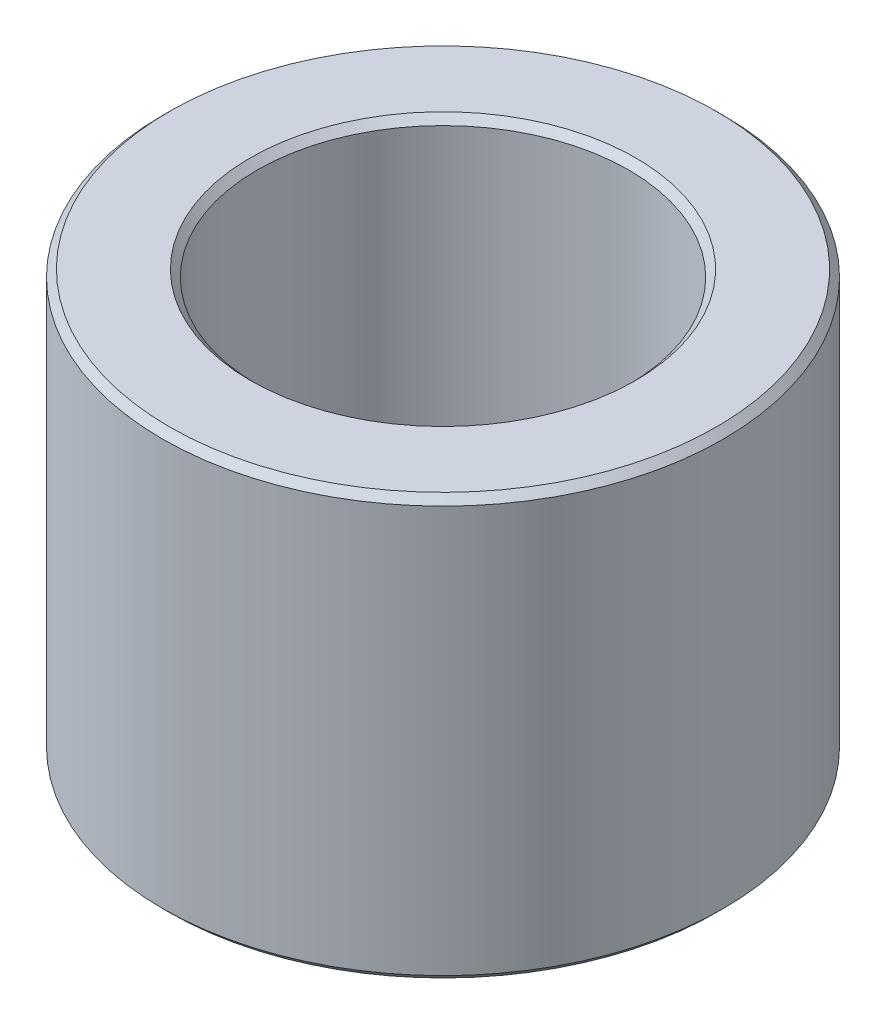
from build123d import *

# Parameters (mm, degrees)
SKETCH1_R           = 8
SKETCH1_R_2         = 5.3
BOSS_EXTRUDE1_DEPTH = 12
CHAMFER1_SIZE       = 0.2


with BuildPart() as part:
    # Sketch1 → Boss-Extrude1 (new body)
    with BuildSketch(Plane(origin=(0, 0, 0), x_dir=(1, 0, 0), z_dir=(0, 1, 0))):
        with Locations(Location((0, 0, 0), (0, 0, 270))):
            Circle(SKETCH1_R)
        with Locations(Location((0, 0, 0), (0, 0, 270))):
            Circle(SKETCH1_R_2, mode=Mode.SUBTRACT)
    extrude(amount=BOSS_EXTRUDE1_DEPTH)

    # Chamfer1
    chamfer1_edges = [part.edges().sort_by_distance(p)[0] for p in [
        (0, 0, -8),
        (0, 12, -8),
        (0, 0, -5.3),
        (0, 12, -5.3),
    ]]
    chamfer(chamfer1_edges, length=CHAMFER1_SIZE)


solid = part.part
